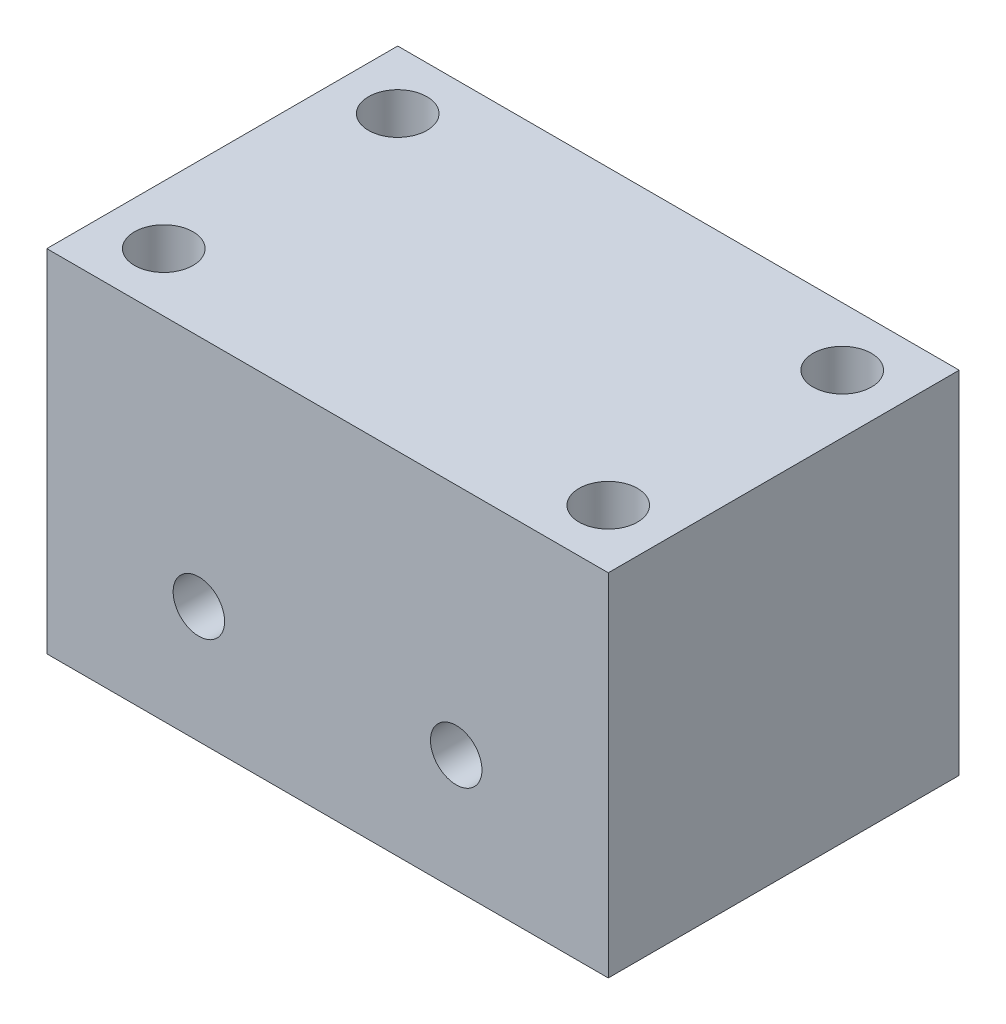
SolidWorks part; units mm, degrees
ref_plane "前视基准面" through (0, 0, 0) normal (0, 0, 1) x (1, 0, 0)
ref_plane "上视基准面" through (0, 0, 0) normal (0, 1, 0) x (1, 0, 0)
ref_plane "右视基准面" through (0, 0, 0) normal (1, 0, 0) x (0, 0, -1)
sketch "草图1" plane through (0, 0, 0) normal (0, 0, 1) x (1, 0, 0)
  line L1 (-24.5455, 16.5273) -> (23.4545, 16.5273)
  line L2 (-24.5455, 16.5273) -> (-24.5455, -13.4727)
  line L3 (-24.5455, -13.4727) -> (23.4545, -13.4727)
  line L4 (23.4545, 16.5273) -> (23.4545, -13.4727)
  dimension "D1" = 48
  dimension "D2" = 30
extrude "凸台-拉伸1" add sketch "草图1" along normal blind 30
sketch "草图2" plane through (0, 0, 0) normal (0, 0, -1) x (-1, 0, 0)
  line L0 (24.5455, -13.4727) -> (-23.4545, -13.4727) construction
  line L1 (-13.4545, -13.4727) -> (14.5455, -13.4727)
  line L2 (-13.4545, -13.4727) -> (-13.4545, 1.5273)
  line L3 (-13.4545, 1.5273) -> (14.5455, 1.5273)
  line L4 (14.5455, -13.4727) -> (14.5455, 1.5273)
  line L5 (-23.4545, -13.4727) -> (-23.4545, 16.5273) construction
  dimension "D1" = 28
  dimension "D2" = 15
  dimension "D3" = 10
extrude "切除-拉伸1" cut sketch "草图2" against normal blind 20
sketch "草图3" plane through (0, 0, 20) normal (0, 0, -1) x (-1, 0, 0)
  line L0 (14.5455, 1.5273) -> (-13.4545, 1.5273) construction
  line L1 (-13.4545, 1.5273) -> (-13.4545, -13.4727) construction
  line L2 (14.5455, 1.5273) -> (-13.4545, 1.5273) construction
  line L3 (14.5455, -13.4727) -> (14.5455, 1.5273) construction
  circle A0 centre (-10.4545, -3.4727) radius 2.2
  circle A1 centre (11.5455, -3.4727) radius 2.2
  dimension "D5" = 4.4
  dimension "D6" = 4.4
  dimension "D1" = 5
  dimension "D2" = 3
  dimension "D3" = 5
  dimension "D4" = 3
extrude "切除-拉伸2" cut sketch "草图3" against normal blind 20
sketch "草图4" plane through (0, -13.4727, 0) normal (0, -1, 0) x (1, 0, 0)
  line L0 (-24.5455, 30) -> (23.4545, 30) construction
  line L1 (-24.5455, 30) -> (-24.5455, 0) construction
  line L2 (-24.5455, 0) -> (-14.5455, 0) construction
  line L3 (23.4545, 30) -> (23.4545, 0) construction
  line L4 (13.4545, 0) -> (23.4545, 0) construction
  circle A1 centre (-19.5455, 5) radius 2.5
  circle A2 centre (-19.5455, 25) radius 2.5
  circle A3 centre (18.4545, 25) radius 2.5
  circle A4 centre (18.4545, 5) radius 2.5
  dimension "D9" = 5
  dimension "D10" = 5
  dimension "D11" = 5
  dimension "D12" = 5
  dimension "D1" = 5
  dimension "D2" = 5
  dimension "D3" = 5
  dimension "D4" = 5
  dimension "D5" = 5
  dimension "D6" = 5
  dimension "D7" = 5
  dimension "D8" = 5
extrude "切除-拉伸3" cut sketch "草图4" against normal up to surface (30 mm away) up to face at (-0.5455, 16.5273, 15)
